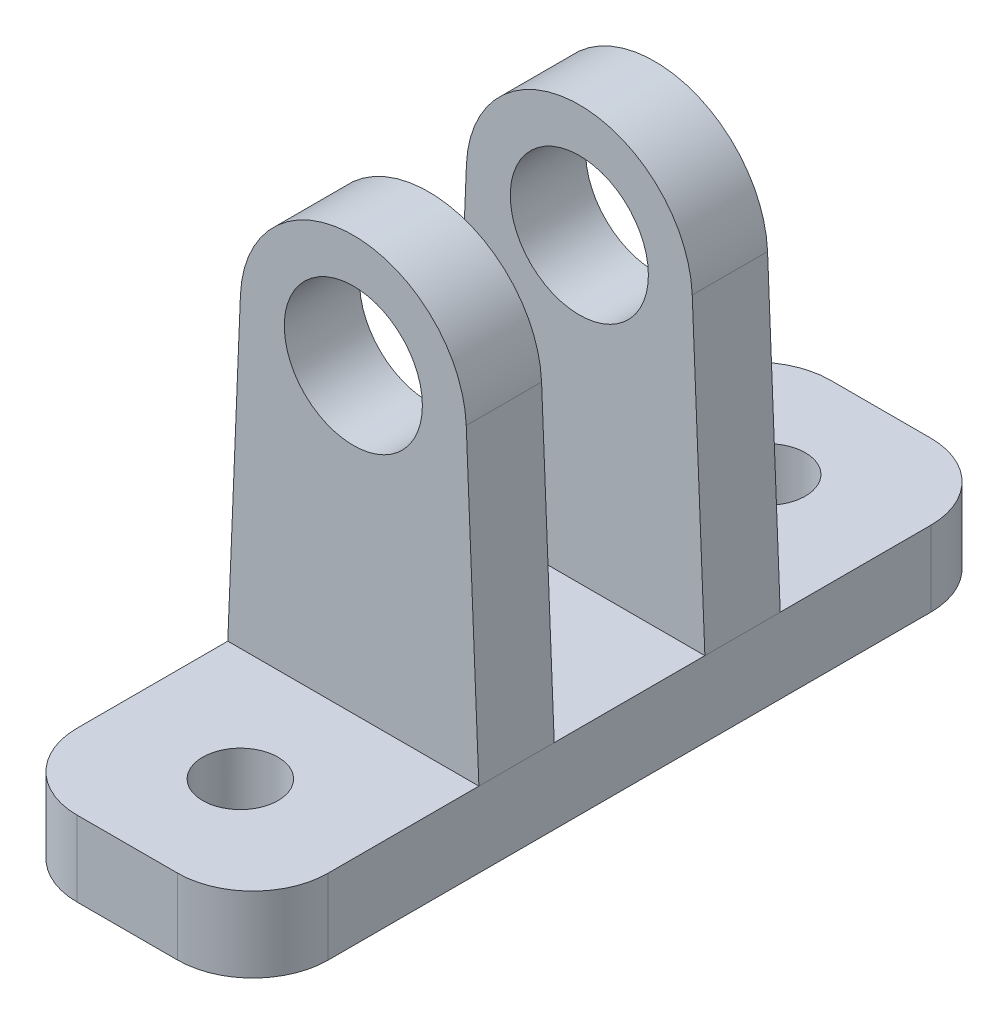
from build123d import *

# Parameters (mm, degrees)
SKETCH_1_W           = 100
SKETCH_1_H           = 120
BOSS_EXTRUDE_1_DEPTH = 30
SKETCH_2_R           = 27.5
BOSS_EXTRUDE_2_DEPTH = 30
SKETCH_4_W           = 15
SKETCH_4_H           = 30
BOSS_EXTRUDE_3_DEPTH = 30
SKETCH_5_W           = 100
SKETCH_5_H           = 300
SKETCH_5_R           = 15
BOSS_EXTRUDE_4_DEPTH = 30
FILLET_1_R           = 30


with BuildPart() as part:
    # Sketch 1 → Boss-Extrude 1 (new body)
    with BuildSketch(Plane(origin=(0, 0, 0), x_dir=(1, 0, 0), z_dir=(0, 1, 0))):
        Rectangle(SKETCH_1_W, SKETCH_1_H)
    extrude(amount=BOSS_EXTRUDE_1_DEPTH)

    # Sketch 2 → Boss-Extrude 2 (add)
    with BuildSketch(Plane.XY.offset(60)):
        with BuildLine():
            Line((-44.961585181, 151.858993825), (-50, 30))
            Line((-50, 30), (50, 30))
            Line((50, 30), (44.961585181, 151.858993825))
            ThreePointArc((44.961585181, 151.858993825), (0, 195), (-44.961585181, 151.858993825))
        make_face()
        with Locations((0, 150)):
            Circle(SKETCH_2_R, mode=Mode.SUBTRACT)
    boss_extrude_2 = extrude(amount=-BOSS_EXTRUDE_2_DEPTH)

    # Sketch 4 → Boss-Extrude 3 (add)
    with BuildSketch(Plane.XY.offset(60)):
        with Locations((0, 15)):
            Rectangle(SKETCH_4_W, SKETCH_4_H)
    boss_extrude_3 = extrude(amount=BOSS_EXTRUDE_3_DEPTH)

    # Mirror 1: Boss-Extrude 2, Boss-Extrude 3 across plane
    add(boss_extrude_2.mirror(Plane.XY))
    add(boss_extrude_3.mirror(Plane.XY))

    # Sketch 5 → Boss-Extrude 4 (add)
    with BuildSketch(Plane.XZ):
        Rectangle(SKETCH_5_W, SKETCH_5_H)
        with Locations(Location((0, -105, 0), (0, 0, 270))):
            Circle(SKETCH_5_R, mode=Mode.SUBTRACT)
        with Locations(Location((0, 105, 0), (0, 0, 270))):
            Circle(SKETCH_5_R, mode=Mode.SUBTRACT)
    extrude(amount=-BOSS_EXTRUDE_4_DEPTH)

    # Fillet 1
    fillet_1_edges = [part.edges().sort_by_distance(p)[0] for p in [
        (-50, 15, -150),
        (50, 15, 150),
        (50, 15, -150),
        (-50, 15, 150),
    ]]
    fillet(fillet_1_edges, radius=FILLET_1_R)


solid = part.part
